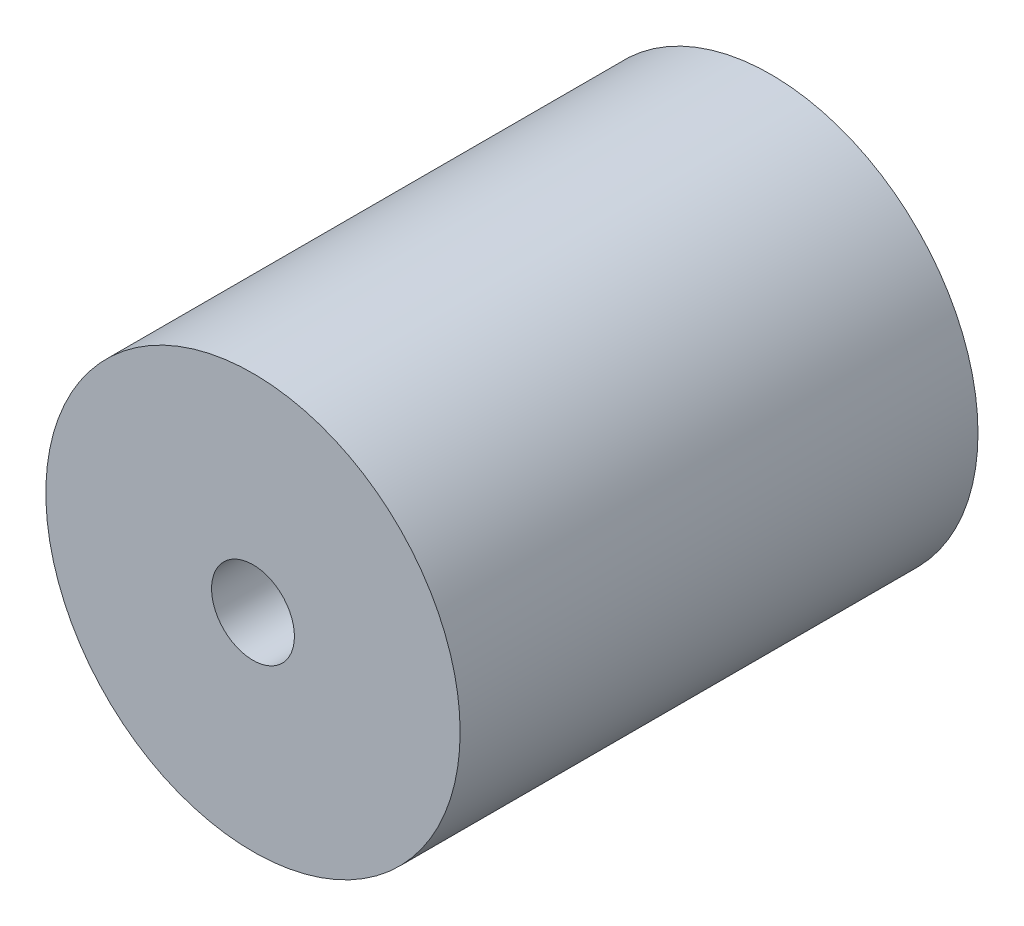
SolidWorks part; units mm, degrees
ref_plane "前视基准面" through (0, 0, 0) normal (0, 0, 1) x (1, 0, 0)
ref_plane "上视基准面" through (0, 0, 0) normal (0, 1, 0) x (1, 0, 0)
ref_plane "右视基准面" through (0, 0, 0) normal (1, 0, 0) x (0, 0, -1)
sketch "草图1" plane through (0, 0, 0) normal (0, 0, 1) x (1, 0, 0)
  circle A0 centre (0, 0) radius 20
  circle A1 centre (0, 0) radius 4
  dimension "D1" = 40
  dimension "D2" = 8
extrude "凸台-拉伸1" add sketch "草图1" along normal blind 50
